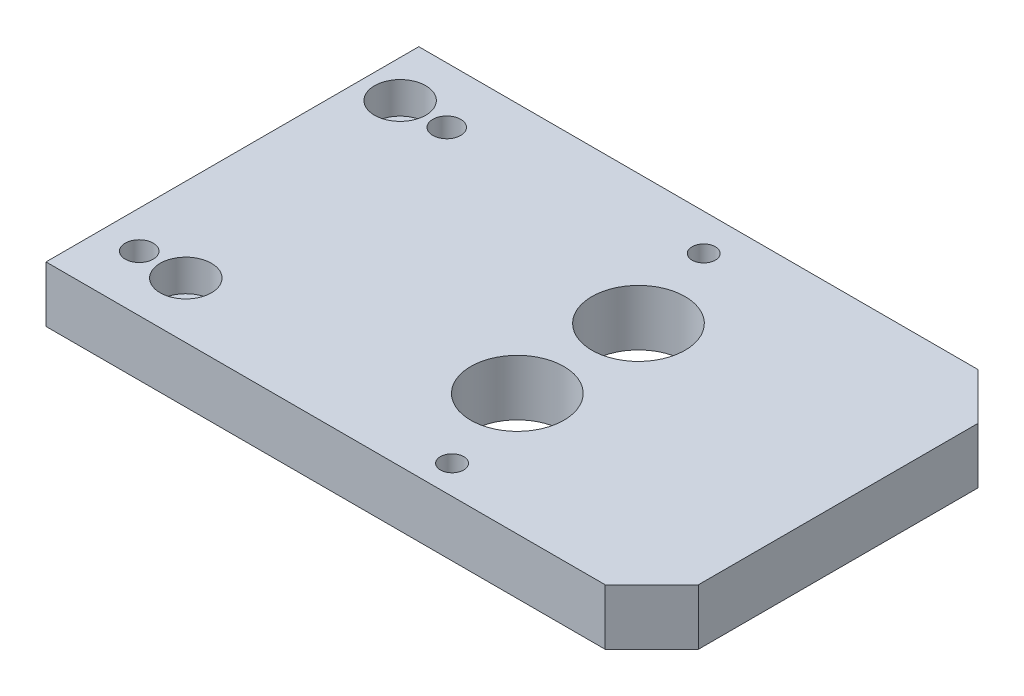
from build123d import *

# Parameters (mm, degrees)
SKETCH1_W                                            = 130
SKETCH1_H                                            = 80
BOSS_EXTRUDE1_DEPTH                                  = 12
CHAMFER1_SIZE                                        = 10
CBORE_FOR_M6_HEXAGON_SOCKET_HEAD_CAP_SCR_D           = 6.6
CBORE_FOR_M6_HEXAGON_SOCKET_HEAD_CAP_SCR_CBORE_D     = 11
CBORE_FOR_M6_HEXAGON_SOCKET_HEAD_CAP_SCR_CBORE_DEPTH = 6.8
F_6_0MM_DOWEL_HOLE_1_D                               = 6
F_20_0MM_DOWEL_HOLE_1_D                              = 20
SKETCH17_R                                           = 2.5
CUT_EXTRUDE1_DEPTH                                   = 154.114336363


with BuildPart() as part:
    # Sketch1 → Boss-Extrude1 (new body)
    with BuildSketch(Plane(origin=(0, 0, 0), x_dir=(1, 0, 0), z_dir=(0, 1, 0))):
        with Locations((65, 40)):
            Rectangle(SKETCH1_W, SKETCH1_H)
    extrude(amount=BOSS_EXTRUDE1_DEPTH)

    # Chamfer1
    chamfer1_edges = [part.edges().sort_by_distance(p)[0] for p in [
        (130, 6, -80),
        (130, 6, 0),
    ]]
    chamfer(chamfer1_edges, length=CHAMFER1_SIZE)

    # CBORE for M6 Hexagon socket head cap screws1 (through all)
    with Locations(Plane(origin=(8, 12, -68), x_dir=(0, 0, 1), z_dir=(0, 1, 0))):
        with Locations((0, 0), (56, 10)):
            CounterBoreHole(CBORE_FOR_M6_HEXAGON_SOCKET_HEAD_CAP_SCR_D / 2, CBORE_FOR_M6_HEXAGON_SOCKET_HEAD_CAP_SCR_CBORE_D / 2, CBORE_FOR_M6_HEXAGON_SOCKET_HEAD_CAP_SCR_CBORE_DEPTH)

    # Ø6.0mm dowel hole 1 (through all)
    with Locations(Plane(origin=(18, 12, -68), x_dir=(0, 0, 1), z_dir=(0, 1, 0))):
        with Locations((0, 0), (56, -10)):
            Hole(F_6_0MM_DOWEL_HOLE_1_D / 2)

    # Ø20.0mm dowel hole 1 (through all)
    with Locations(Plane(origin=(0, 0, 0), x_dir=(-1, 0, 0), z_dir=(0, -1, 0))):
        with Locations((-75, 52.142135624), (-75, 26.142135624)):
            Hole(F_20_0MM_DOWEL_HOLE_1_D / 2)

    # Sketch17 → Cut-Extrude1 (cut, through all)
    with BuildSketch(Plane(origin=(0, 12, 0), x_dir=(1, 0, 0), z_dir=(0, 1, 0))):
        with Locations(Location((81, 6.142135624, 0), (0, 0, 270))):
            Circle(SKETCH17_R)
        with Locations(Location((69, 72.142135624, 0), (0, 0, 270))):
            Circle(SKETCH17_R)
    extrude(amount=-CUT_EXTRUDE1_DEPTH, mode=Mode.SUBTRACT)


solid = part.part
